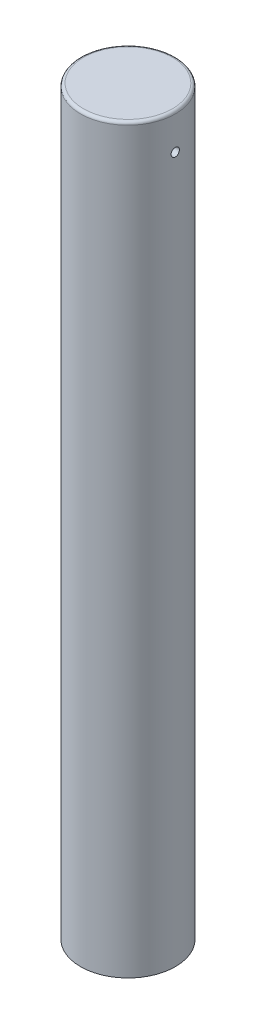
SolidWorks part; units mm, degrees
ref_plane "Front" through (0, 0, 0) normal (0, 0, 1) x (1, 0, 0)
ref_plane "Top" through (0, 0, 0) normal (0, 1, 0) x (1, 0, 0)
ref_plane "Side view" through (0, 0, 0) normal (1, 0, 0) x (0, 0, -1)
sketch "Sketch1" plane through (0, 0, 0) normal (0, 0, 1) x (1, 0, 0)
  line L0 (0, 38.2054) -> (0, -37.8043) construction
  line L1 (0, -37.8043) -> (-8, -37.8043)
  line L2 (-8, -37.8043) -> (-8, 86.6957)
  line L3 (-7.5, 87.1957) -> (0, 87.1957)
  line L4 (0, 87.1957) -> (0, -37.8043)
  arc A0 (-8, 86.6957) -> (-7.5, 87.1957) centre (-7.5, 86.6957) cw
  dimension "D3" = 0.5
  dimension "D1" = 8
  dimension "D2" = 125
revolve "Revolution1" add sketch "Sketch1" angle 360 about L0
sketch "Sketch2" plane through (0, 0, 0) normal (0, 0, 1) x (1, 0, 0)
  line L0 (8, 86.6957) -> (8, 81.1137) construction
  line L1 (0, 81.1137) -> (0, 84.9999) construction
  line L2 (8, -37.8043) -> (8, 86.6957) construction
  line L3 (8, 81.1137) -> (-8, 81.1137) construction
  line L4 (-8, 86.6957) -> (-8, -37.8043) construction
  line L5 (8, 81.8137) -> (6.5, 81.8137)
  line L8 (8, 81.1137) -> (8, 81.8137)
  line L9 (-8, 81.1137) -> (-8, 81.8137)
  line L11 (-8, 81.8137) -> (-6.5, 81.8137)
  line L12 (5.8, 81.1137) -> (8, 81.1137)
  line L13 (-5.8, 81.1137) -> (-8, 81.1137)
  arc A2 (6.5, 81.8137) -> (5.8, 81.1137) centre (6.5, 81.1137) ccw
  arc A3 (-6.5, 81.8137) -> (-5.8, 81.1137) centre (-6.5, 81.1137) cw
  dimension "D1" = 1.5
  dimension "D2" = 0.7
revolve "Cut-Revolve1" cut sketch "Sketch2" angle 360 about L3
hole_wizard "Clearance hole for M1.61" positions "Sketch5" profile "Sketch6" hole size "M1.6" standard "Ansi Metric"
sketch "Sketch5" plane through (0, -37.8043, 0) normal (0, -1, 0) x (-1, 0, 0)
  point P0 (0, 0)
sketch "Sketch6" plane through (0, -37.8043, 0) normal (1, 0, 0) x (0, 0, -1)
  line L0 (0, 0) -> (0, 8.5408)
  line L1 (0, 8.5408) -> (0.9, 8)
  line L2 (0.9, 8) -> (0.9, 0)
  line L5 (0.9, 0) -> (0, 0)
  line L10 (0, 8.5408) -> (-0.9, 8) construction
  line L11 (0, -6.35) -> (0, 107.95) construction
  dimension "Diámetro de taladro" = 1.8
  dimension "Profundidad de taladro" = 8
  dimension "Ángulo de perforador" = 118
